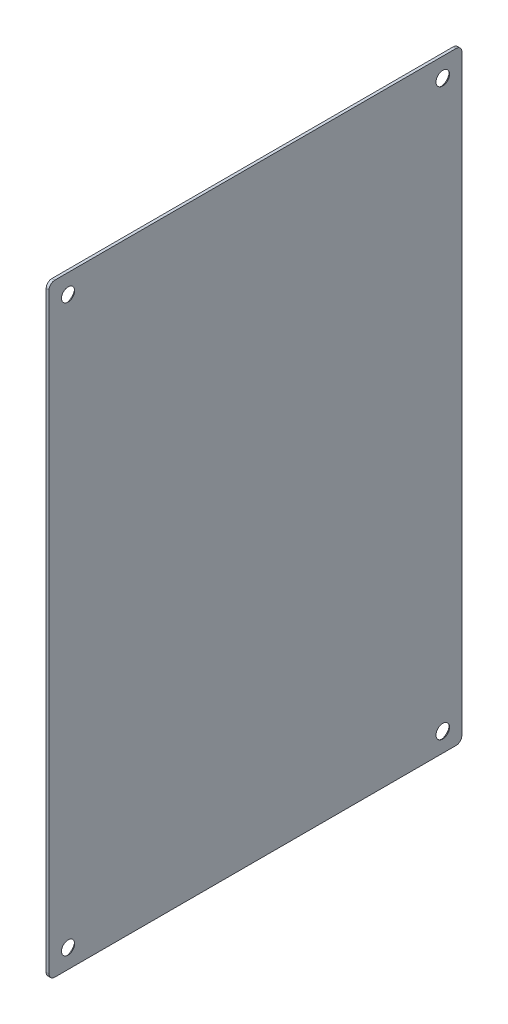
SolidWorks part; units mm, degrees
ref_plane "前视基准面" through (0, 0, 0) normal (0, 0, 1) x (1, 0, 0)
ref_plane "上视基准面" through (0, 0, 0) normal (0, 1, 0) x (1, 0, 0)
ref_plane "右视基准面" through (0, 0, 0) normal (1, 0, 0) x (0, 0, -1)
ref_plane "基准面4" through (2615.9295, 0, 0) normal (-1, 0, 0) x (0, -1, 0)
sketch "草图1" plane through (2615.9295, 0, 0) normal (-1, 0, 0) x (0, -1, 0)
  line L0 (-1369.3, 299.1446) -> (-1369.3, 82.6446)
  line L1 (-1369.3, 82.6446) -> (-1052.7, 82.6446)
  line L2 (-1052.7, 82.6446) -> (-1052.7, 299.1446)
  line L3 (-1052.7, 299.1446) -> (-1369.3, 299.1446)
extrude "凸台-拉伸1" add sketch "草图1" against normal blind 1.5
hole_wizard "孔1" positions "草图3" profile "草图2" legacy
sketch "草图3" plane through (2615.9295, 0, 0) normal (-1, 0, 0) x (0, 0, 1)
  point P0 (289.1446, 1062.7)
  point P1 (289.1446, 1359.3)
sketch "草图2" plane through (2615.9295, 1062.7, 289.1446) normal (0, 1, 0) x (0, 0, 1)
  line L0 (0, 0) -> (0, 1.5)
  line L1 (0, 1.5) -> (3.45, 1.5)
  line L2 (3.45, 1.5) -> (4.95, 0)
  line L3 (4.95, 0) -> (0, 0)
  line L4 (0, 110) -> (0, -10) construction
  dimension "次要直径" = 6.9
  dimension "深度" = 1.5
  dimension "主要直径" = 9.9
hole_wizard "Ø7.1 (7.1) 直径孔1" positions "草图5" profile "草图4" hole size "Ø7.1" standard "ANSI Metric"
sketch "草图5" plane through (2615.9295, 0, 0) normal (-1, 0, 0) x (0, 0, 1)
  point P0 (92.6446, 1359.3)
  point P1 (92.6446, 1062.7)
sketch "草图4" plane through (2615.9295, 1359.3, 92.6446) normal (0, 1, 0) x (0, 0, 1)
  line L0 (0, 0) -> (0, 1.5)
  line L1 (0, 1.5) -> (3.55, 1.5)
  line L2 (3.55, 1.5) -> (3.55, 1.4)
  line L3 (3.55, 1.4) -> (4.95, 0)
  line L5 (4.95, 0) -> (0, 0)
  line L6 (-3.55, 1.4) -> (-4.95, 0) construction
  line L11 (0, -6.35) -> (0, 107.95) construction
  dimension "通孔孔直径" = 7.1
  dimension "通孔孔深度" = 1.5
  dimension "近端锥形沉头孔直径" = 9.9
  dimension "近端锥形沉头孔角度" = 90
fillet "圆角1" radius 3 4 edges at (2616.6795, 1369.3, 82.6446) (2616.6795, 1052.7, 82.6446) (2616.6795, 1369.3, 299.1446) (2616.6795, 1052.7, 299.1446)
